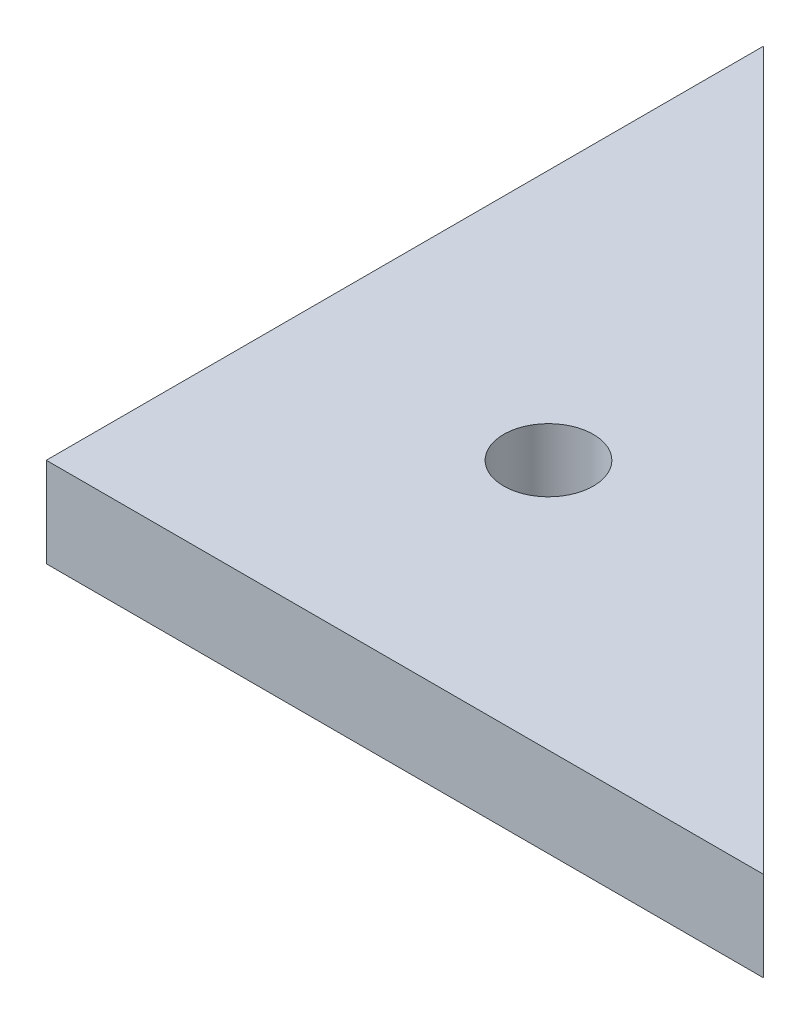
SolidWorks part; units mm, degrees
ref_plane "前视基准面" through (0, 0, 0) normal (0, 0, 1) x (1, 0, 0)
ref_plane "上视基准面" through (0, 0, 0) normal (0, 1, 0) x (1, 0, 0)
ref_plane "右视基准面" through (0, 0, 0) normal (1, 0, 0) x (0, 0, -1)
sketch "草图1" plane through (0, 0, 0) normal (0, 1, 0) x (1, 0, 0)
  line L0 (0, 40) -> (0, 0)
  line L1 (0, 0) -> (40, 0)
  line L2 (40, 0) -> (0, 40)
  dimension "D1" = 40
  dimension "D2" = 40
extrude "凸台-拉伸1" add sketch "草图1" along normal blind 5
hole_wizard "M6 螺纹孔1" positions "草图2" profile "草图3" tap size "M6" standard "GB"
sketch "草图2" plane through (0, 5, 0) normal (0, 1, 0) x (1, 0, 0)
  line L0 (0, 40) -> (0, 0) construction
  line L1 (0, 0) -> (40, 0) construction
  point P0 (14, 14)
  dimension "D1" = 14
  dimension "D2" = 14
sketch "草图3" plane through (14, 5, -14) normal (1, 0, 0) x (0, 0, 1)
  line L0 (0, 0) -> (0, 16.5022)
  line L1 (0, 16.5022) -> (2.5, 15)
  line L2 (2.5, 15) -> (2.5, 0)
  line L5 (2.5, 0) -> (0, 0)
  line L10 (0, 16.5022) -> (-2.5, 15) construction
  line L11 (0, -6.35) -> (0, 107.95) construction
  dimension "螺纹孔钻头直径" = 5
  dimension "螺纹孔钻头深度" = 15
  dimension "导头角度" = 118
cosmetic thread "孔螺蚊线1" parameters "D1"=5, "D2"=6
